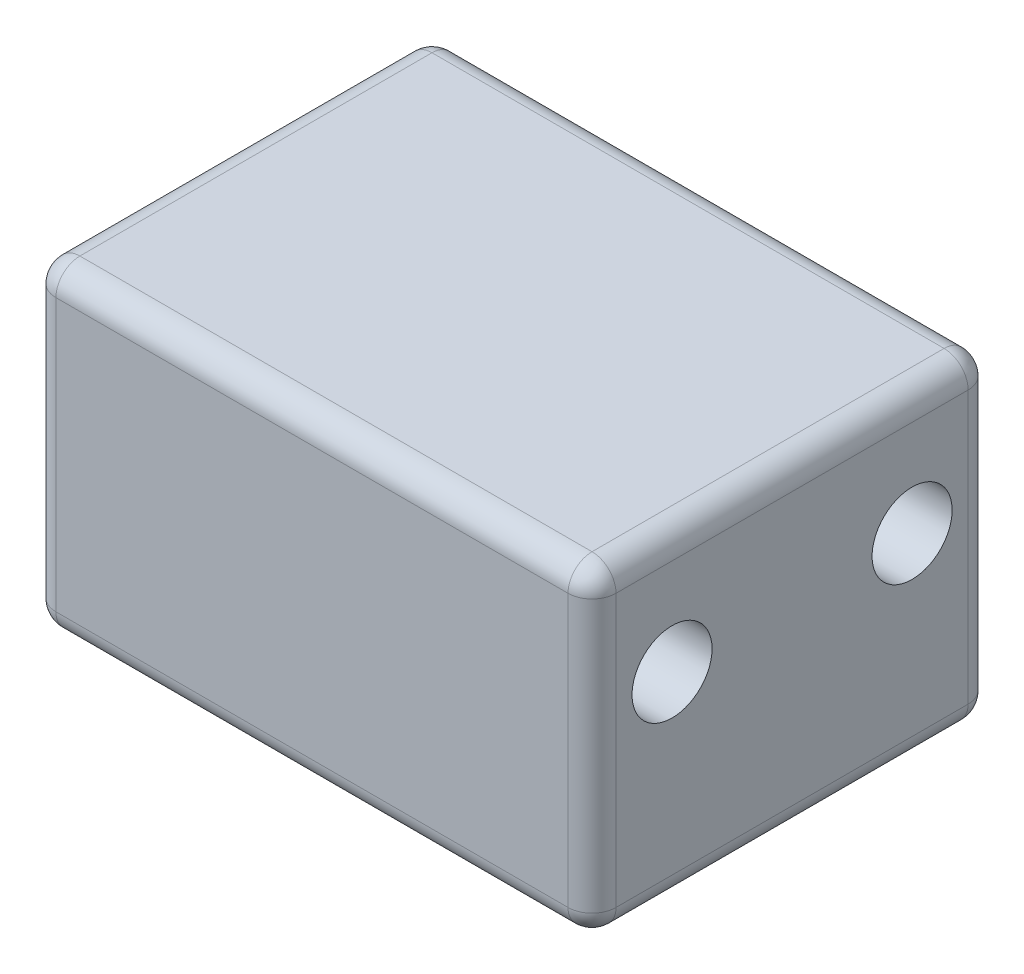
from build123d import *

# Parameters (mm, degrees)
SKETCH1_W           = 70
SKETCH1_H           = 50
BOSS_EXTRUDE1_DEPTH = 40
SKETCH2_R           = 5
CUT_EXTRUDE1_DEPTH  = 95.868329805
SKETCH3_R           = 6
CUT_EXTRUDE2_DEPTH  = 35
SKETCH4_R           = 10.5
CUT_EXTRUDE3_DEPTH  = 7
FILLET1_R           = 3


with BuildPart() as part:
    # Sketch1 → Boss-Extrude1 (new body)
    with BuildSketch(Plane(origin=(0, 0, 0), x_dir=(1, 0, 0), z_dir=(0, 1, 0))):
        with Locations((35, 25)):
            Rectangle(SKETCH1_W, SKETCH1_H)
    extrude(amount=BOSS_EXTRUDE1_DEPTH)

    # Sketch2 → Cut-Extrude1 (cut, through all)
    with BuildSketch(Plane(origin=(70, 0, 0), x_dir=(0, 0, -1), z_dir=(1, 0, 0))):
        with Locations((40, 25)):
            Circle(SKETCH2_R)
        with Locations((10, 25)):
            Circle(SKETCH2_R)
    extrude(amount=-CUT_EXTRUDE1_DEPTH, mode=Mode.SUBTRACT)

    # Sketch3 → Cut-Extrude2 (cut)
    with BuildSketch(Plane.XZ):
        with Locations(Location((60, -25, 0), (0, 0, 270))):
            Circle(SKETCH3_R)
    extrude(amount=-CUT_EXTRUDE2_DEPTH, mode=Mode.SUBTRACT)

    # Sketch4 → Cut-Extrude3 (cut)
    with BuildSketch(Plane.XZ):
        with Locations(Location((15, -25, 0), (0, 0, 270))):
            Circle(SKETCH4_R)
    extrude(amount=-CUT_EXTRUDE3_DEPTH, mode=Mode.SUBTRACT)

    # Fillet1
    fillet1_edges = [part.edges().sort_by_distance(p)[0] for p in [
        (70, 40, -25),
        (35, 40, -50),
        (0, 40, -25),
        (35, 0, -50),
        (70, 0, -25),
        (35, 0, 0),
        (0, 0, -25),
        (35, 40, 0),
        (0, 20, -50),
        (70, 20, -50),
        (70, 20, 0),
        (0, 20, 0),
    ]]
    fillet(fillet1_edges, radius=FILLET1_R)


solid = part.part
